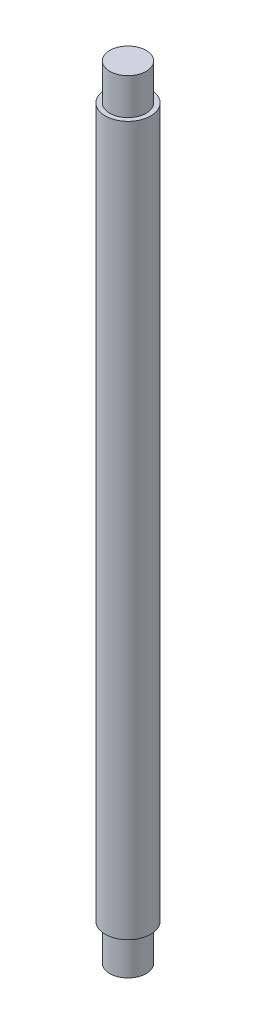
from build123d import *

# Parameters (mm, degrees)
SKETCH1_R           = 5
BOSS_EXTRUDE1_DEPTH = 78
SKETCH2_R           = 4
BOSS_EXTRUDE2_DEPTH = 8


with BuildPart() as part:
    # Sketch1 → Boss-Extrude1 (new, symmetric)
    with BuildSketch(Plane(origin=(0, 0, 0), x_dir=(1, 0, 0), z_dir=(0, 1, 0))):
        with Locations(Location((0, 0, 0), (0, 0, 270))):
            Circle(SKETCH1_R)
    extrude(amount=BOSS_EXTRUDE1_DEPTH, both=True)

    # Sketch2 → Boss-Extrude2 (add)
    with BuildSketch(Plane(origin=(0, 78, 0), x_dir=(1, 0, 0), z_dir=(0, 1, 0))):
        with Locations(Location((0, 0, 0), (0, 0, 270))):
            Circle(SKETCH2_R)
    boss_extrude2 = extrude(amount=BOSS_EXTRUDE2_DEPTH)

    # Mirror1: Boss-Extrude2 across plane
    add(boss_extrude2.mirror(Plane.ZX))


solid = part.part
